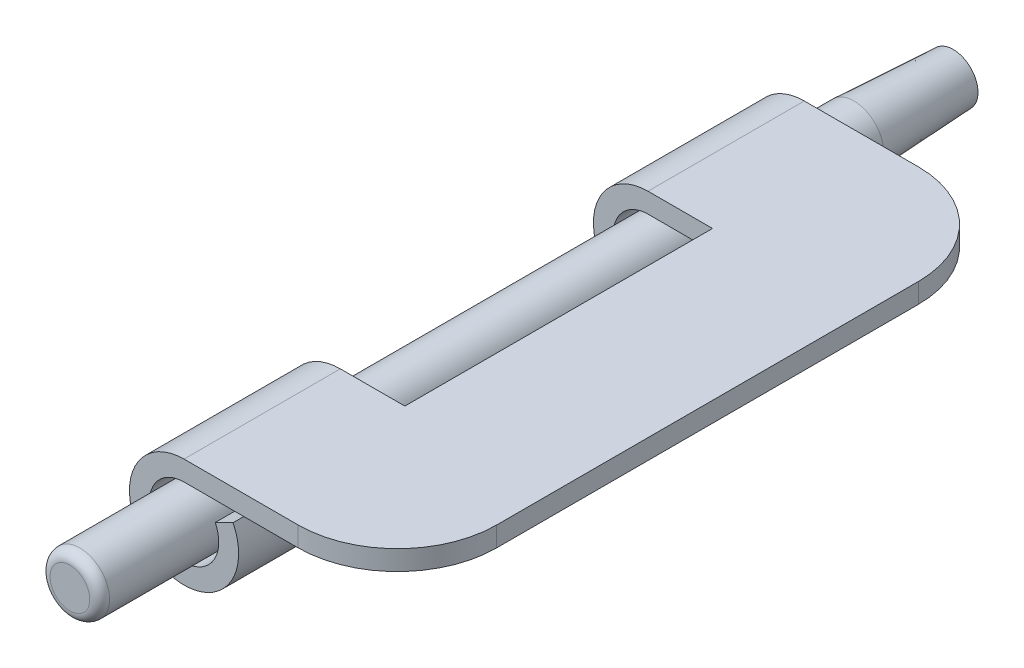
from build123d import *

# Parameters (mm, degrees)
EXTRUDE_5_DEPTH     = 31.25
SKETCH_4_W          = 12
SKETCH_4_H          = 31
CUT_EXTRUDE_1_DEPTH = 40.494461637
SKETCH_6_R          = 3
EXTRUDE_3_DEPTH     = 89
CHAMFER_1_SIZE      = 0.5
CHAMFER_1_SIZE2     = 10
FILLET_1_R          = 10
FILLET_2_R          = 1


with BuildPart() as part:
    # 草图3 → 拉伸-薄壁5 (new, symmetric)
    with BuildSketch(Plane.XY):
        with BuildLine():
            Line((21.5, 0), (0, 0))
            ThreePointArc((0, 0), (-1.852031969, -6.469844707), (3.142998481, -1.960012809))
            Line((3.142998481, -1.960012809), (4.938997613, -1.080020128))
            ThreePointArc((4.938997613, -1.080020128), (-2.910335952, -8.166898826), (0, 2))
            Line((0, 2), (21.5, 2))
            Line((21.5, 2), (21.5, 0))
        make_face()
    extrude(amount=EXTRUDE_5_DEPTH, both=True)

    # 草图4 → 切除-拉伸1 (cut, through all)
    with BuildSketch(Plane(origin=(0, 2, 0), x_dir=(1, 0, 0), z_dir=(0, 1, 0))):
        with Locations((0.5, 0)):
            Rectangle(SKETCH_4_W, SKETCH_4_H)
    extrude(amount=-CUT_EXTRUDE_1_DEPTH, mode=Mode.SUBTRACT)

    # 圆角1
    fillet_1_edges = [part.edges().sort_by_distance(p)[0] for p in [
        (21.5, 1, 31.25),
        (21.5, 1, -31.25),
    ]]
    fillet(fillet_1_edges, radius=FILLET_1_R)


with BuildPart() as body_2:
    # 草图6 → 凸台-拉伸3 (new body)
    with BuildSketch(Plane.XY.offset(42.75)):
        with Locations((0, -3.5)):
            Circle(SKETCH_6_R)
    extrude(amount=-EXTRUDE_3_DEPTH)

    # 倒角1
    chamfer_1_edges = [body_2.edges().sort_by_distance(p)[0] for p in [
        (-3, -3.5, -46.25),
    ]]
    chamfer_1_side = [body_2.faces().sort_by_distance(p)[0] for p in [
        (0, -3.5, -46.25),
    ]]
    chamfer(chamfer_1_edges, length=CHAMFER_1_SIZE, length2=CHAMFER_1_SIZE2, reference=chamfer_1_side[0])

    # 圆角2
    fillet_2_edges = [body_2.edges().sort_by_distance(p)[0] for p in [
        (-3, -3.5, 42.75),
    ]]
    fillet(fillet_2_edges, radius=FILLET_2_R)


solid = Compound([part.part, body_2.part])
